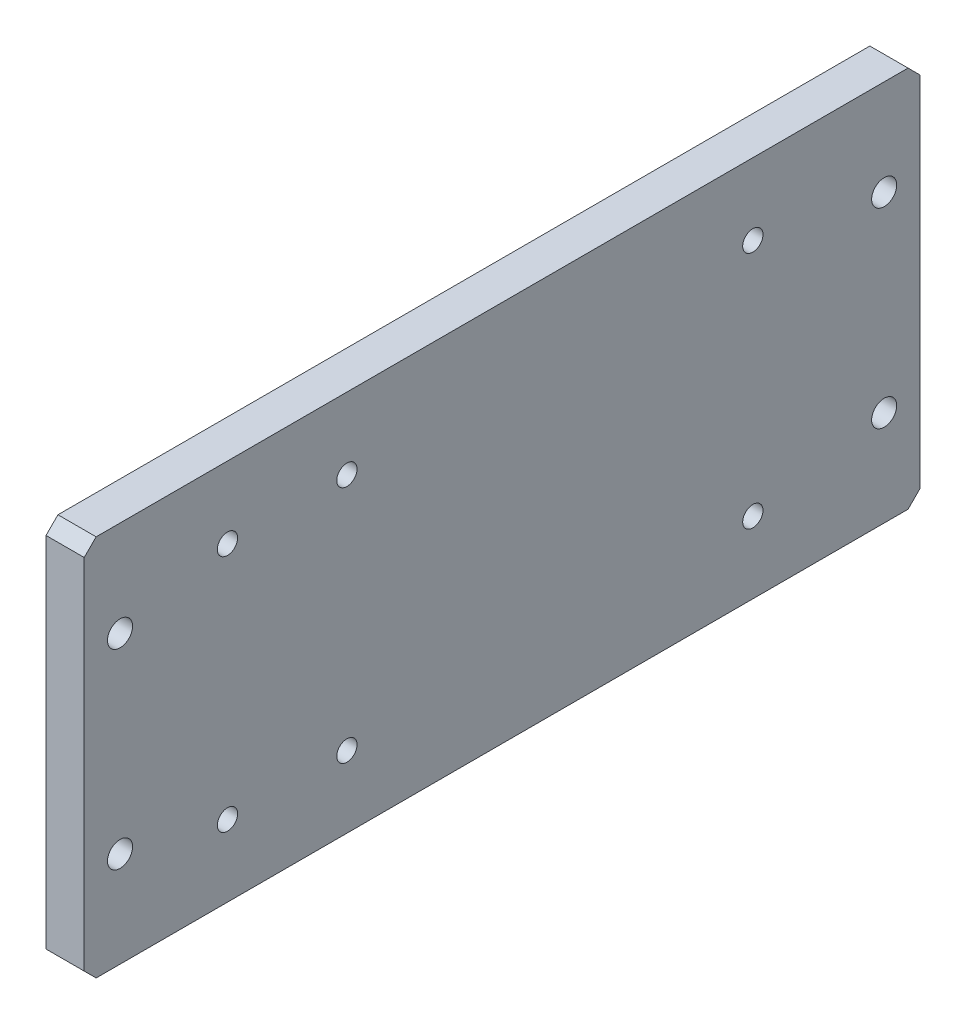
from build123d import *

# Parameters (mm, degrees)
SKETCH_1_W                = 350
SKETCH_1_H                = 160
EXTRUDE_1_DEPTH           = 16
HOLE_WIZARD_M10_1_D       = 8.5
HOLE_WIZARD_10_5_10_5_1_D = 10.5
CHAMFER_1_SIZE            = 5


with BuildPart() as part:
    # 草图1 → 凸台-拉伸1 (new body)
    with BuildSketch(Plane(origin=(0, 0, 0), x_dir=(0, 0, -1), z_dir=(1, 0, 0))):
        Rectangle(SKETCH_1_W, SKETCH_1_H)
    extrude(amount=EXTRUDE_1_DEPTH)

    # M10 螺纹孔1 (through all)
    with Locations(Plane(origin=(16, 0, 0), x_dir=(0, 0, -1), z_dir=(1, 0, 0))):
        with Locations((-115, 50), (-115, -50), (105, 50), (105, -50), (-65, 50), (-65, -50)):
            Hole(HOLE_WIZARD_M10_1_D / 2)

    # Ø10.5 (10.5) 直径孔1 (through all)
    with Locations(Plane.ZY):
        with Locations((-160, 40), (-160, -40), (160, 40), (160, -40)):
            Hole(HOLE_WIZARD_10_5_10_5_1_D / 2)

    # 倒角1
    chamfer_1_edges = [part.edges().sort_by_distance(p)[0] for p in [
        (8, -80, -175),
        (8, -80, 175),
        (8, 80, 175),
        (8, 80, -175),
    ]]
    chamfer(chamfer_1_edges, length=CHAMFER_1_SIZE)


solid = part.part
